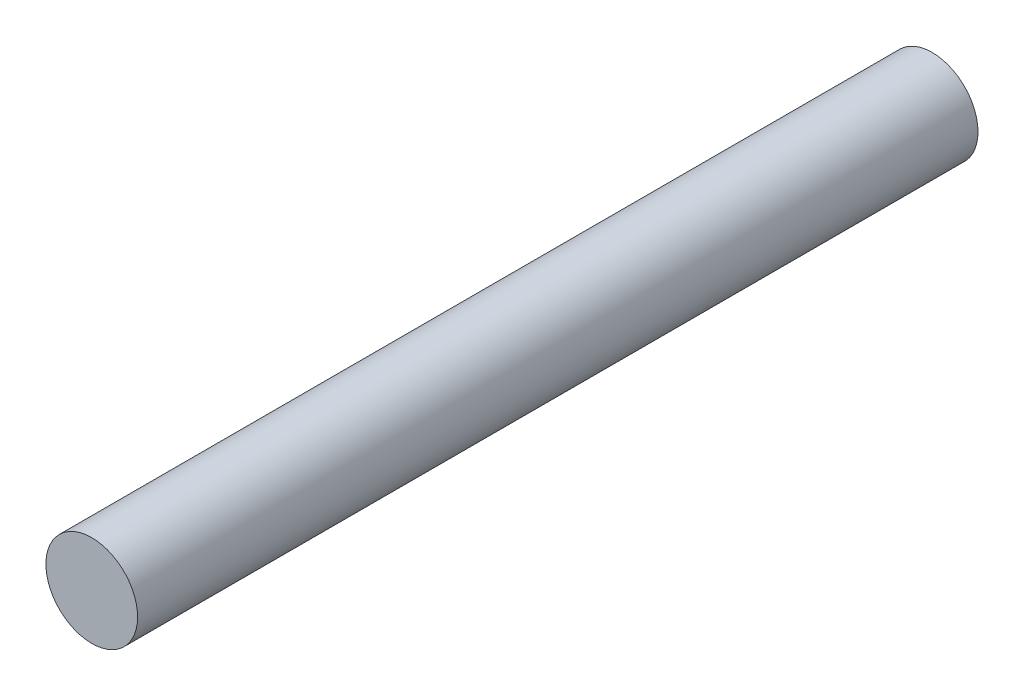
from build123d import *

# Parameters (mm, degrees)
SKETCH_1_R      = 3
EXTRUDE_2_DEPTH = 55


with BuildPart() as part:
    # 草图1 → 凸台-拉伸2 (new body)
    with BuildSketch(Plane.XY):
        Circle(SKETCH_1_R)
    extrude(amount=EXTRUDE_2_DEPTH)


solid = part.part
